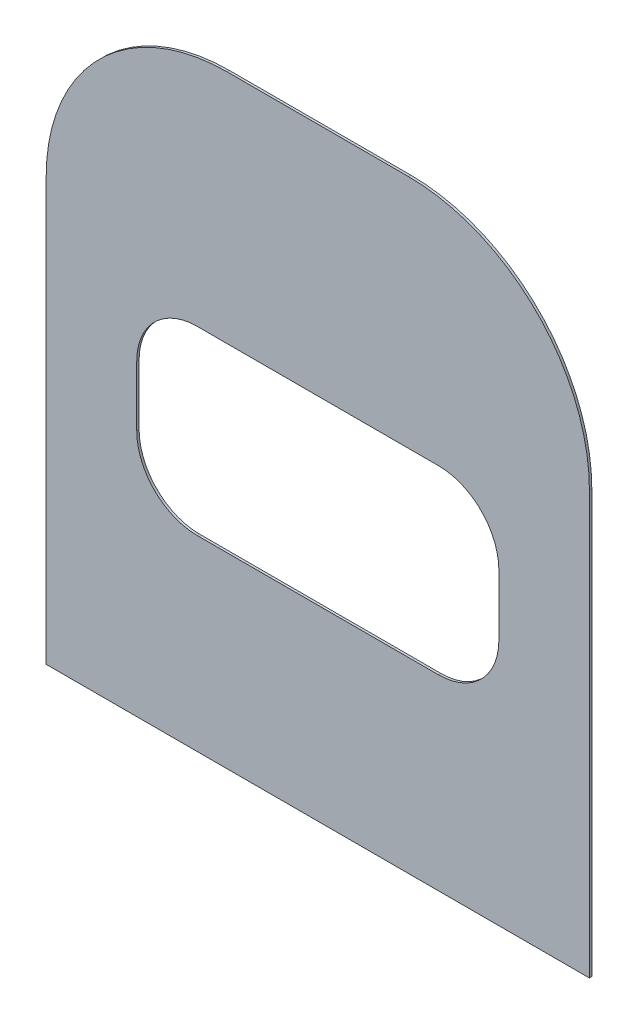
SolidWorks part; units mm, degrees
material "普通碳钢"
ref_plane "Front Plane" through (0, 0, 0) normal (0, 0, 1) x (1, 0, 0)
ref_plane "Top Plane" through (0, 0, 0) normal (0, 1, 0) x (1, 0, 0)
ref_plane "Right Plane" through (0, 0, 0) normal (1, 0, 0) x (0, 0, -1)
sketch "Sketch1" plane through (0, 0, 0) normal (0, 0, 1) x (1, 0, 0)
  line L0 (0, 833.3178) -> (0, -87.1419) construction
  line L2 (-76.2, 508) -> (76.2, 508)
  line L3 (-228.6, 355.6) -> (-228.6, 0)
  line L4 (-228.6, 0) -> (228.6, 0)
  line L5 (228.6, 355.6) -> (228.6, 0)
  line L6 (-101.6, 309.88) -> (101.6, 309.88)
  line L7 (-152.4, 259.08) -> (-152.4, 208.28)
  line L8 (-101.6, 157.48) -> (101.6, 157.48)
  line L9 (152.4, 259.08) -> (152.4, 208.28)
  arc A0 (101.6, 309.88) -> (152.4, 259.08) centre (101.6, 259.08) cw
  arc A1 (-152.4, 208.28) -> (-101.6, 157.48) centre (-101.6, 208.28) ccw
  arc A2 (101.6, 157.48) -> (152.4, 208.28) centre (101.6, 208.28) ccw
  arc A3 (-101.6, 309.88) -> (-152.4, 259.08) centre (-101.6, 259.08) ccw
  arc A4 (76.2, 508) -> (228.6, 355.6) centre (76.2, 355.6) cw
  arc A5 (-76.2, 508) -> (-228.6, 355.6) centre (-76.2, 355.6) ccw
  point P15 (-152.4, 157.48)
  point P18 (152.4, 157.48)
  point P21 (-152.4, 309.88)
  point P26 (-228.6, 508)
  dimension "D6" = 50.8
  dimension "D7" = 152.4
  dimension "D1" = 457.2
  dimension "D2" = 508
  dimension "D3" = 304.8
  dimension "D4" = 152.4
  dimension "D5" = 157.48
extrude "Boss-Extrude1" add sketch "Sketch1" along normal mid plane 2
